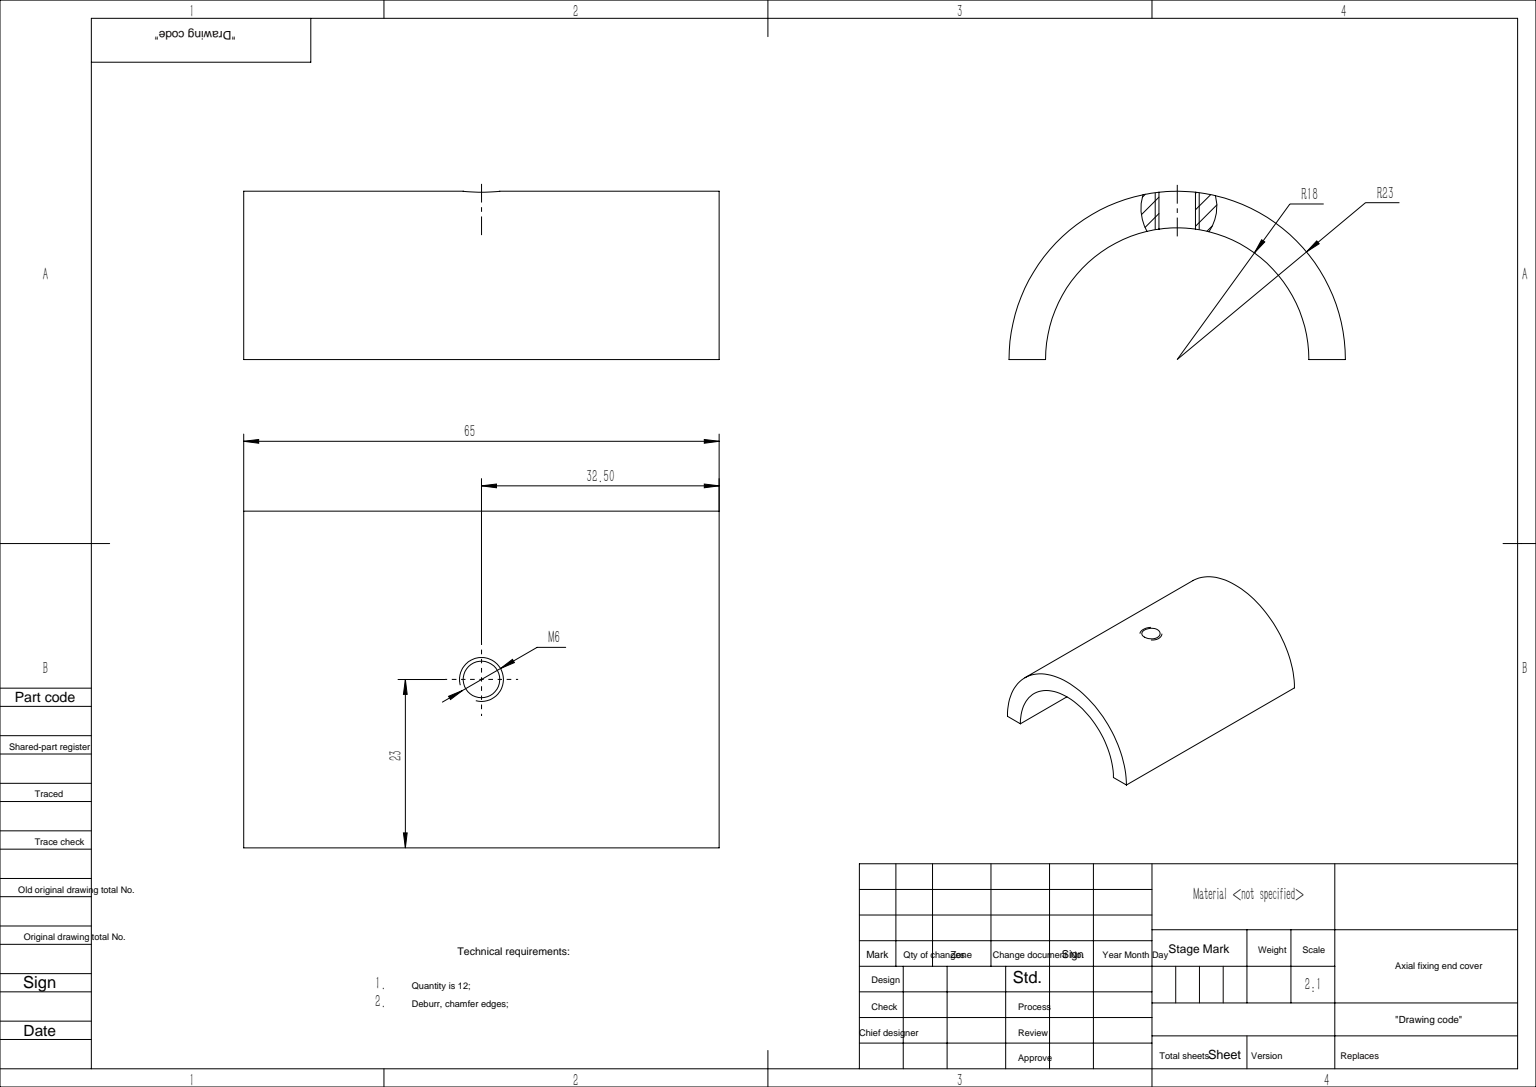
from build123d import *

# Parameters (mm, degrees)
EXTRUDE_1_DEPTH    = 65
HOLE_WIZARD_M6_1_D = 5


with BuildPart() as part:
    # 草图1 → 凸台-拉伸1 (new body)
    with BuildSketch(Plane.XY):
        with BuildLine():
            Line((-23, 0), (-18, 0))
            ThreePointArc((-18, 0), (0, 18), (18, 0))
            Line((18, 0), (23, 0))
            ThreePointArc((23, 0), (0, 23), (-23, 0))
        make_face()
    extrude(amount=-EXTRUDE_1_DEPTH)

    # M6 螺纹孔1 (through all)
    with Locations(Plane(origin=(0, 23, -32.5), x_dir=(1, 0, 0), z_dir=(0, 1, 0))):
        with Locations((0, 0)):
            Hole(HOLE_WIZARD_M6_1_D / 2)


solid = part.part
